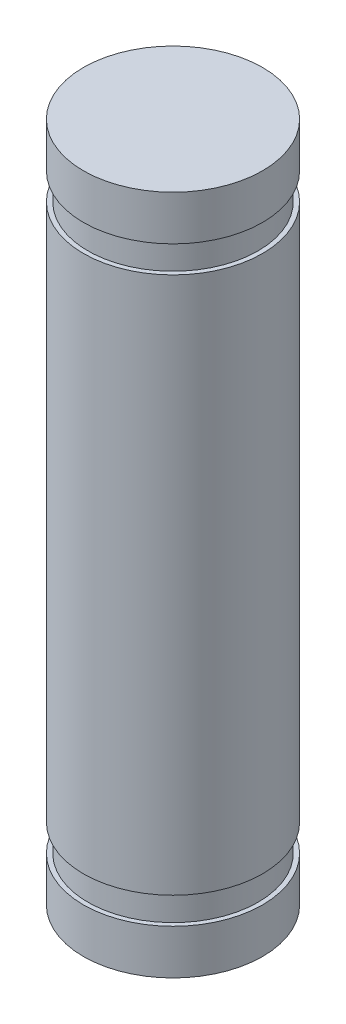
SolidWorks part; units mm, degrees
ref_plane "前视基准面" through (0, 0, 0) normal (0, 0, 1) x (1, 0, 0)
ref_plane "上视基准面" through (0, 0, 0) normal (0, 1, 0) x (1, 0, 0)
ref_plane "右视基准面" through (0, 0, 0) normal (1, 0, 0) x (0, 0, -1)
sketch "草图1" plane through (0, 0, 0) normal (0, 0, 1) x (1, 0, 0)
  line L0 (0, 2.6466) -> (0, 50002.6466) construction
  line L1 (0, 2.6466) -> (2, 2.6466)
  line L2 (2, 2.6466) -> (2, 1.6466)
  line L3 (2, 1.6466) -> (1.9, 1.6466)
  line L4 (1.9, 1.6466) -> (1.9, 1.0466)
  line L5 (1.9, 1.0466) -> (2, 1.0466)
  line L13 (2, 1.0466) -> (2, -10.9534)
  line L14 (2, -10.9534) -> (1.9, -10.9534)
  line L15 (1.9, -10.9534) -> (1.9, -11.5534)
  line L16 (1.9, -11.5534) -> (2, -11.5534)
  line L17 (2, -11.5534) -> (2, -12.5534)
  line L18 (2, -12.5534) -> (0, -12.5534)
  line L19 (0, 2.6466) -> (0, -12.5534)
  dimension "D1" = 2
  dimension "D2" = 1
  dimension "D3" = 0.1
  dimension "D4" = 0.6
  dimension "D5" = 0.1
  dimension "D6" = 12
  dimension "D7" = 0.1
  dimension "D8" = 1
  dimension "D9" = 0.6
revolve "旋转1" add sketch "草图1" angle 360 about L19
